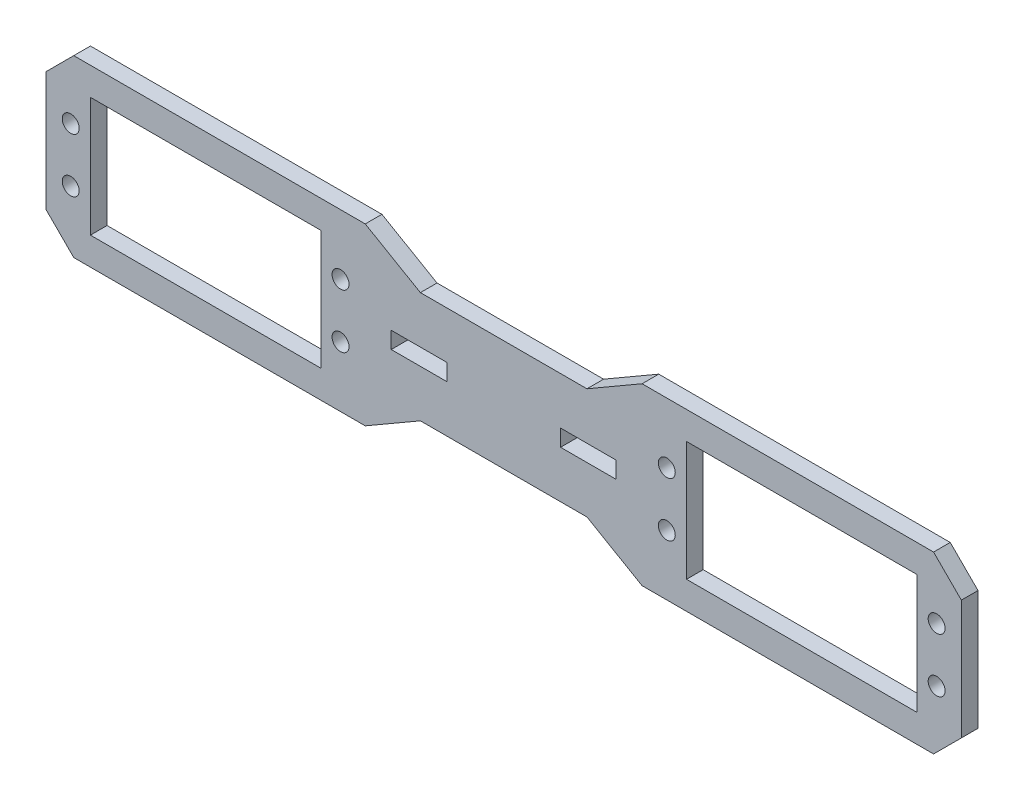
SolidWorks part; units mm, degrees
ref_plane "前视基准面" through (0, 0, 0) normal (0, 0, 1) x (1, 0, 0)
ref_plane "上视基准面" through (0, 0, 0) normal (0, 1, 0) x (1, 0, 0)
ref_plane "右视基准面" through (0, 0, 0) normal (1, 0, 0) x (0, 0, -1)
other "Configuration Table"
sketch "草图1" plane through (0, 0, 0) normal (0, 0, 1) x (1, 0, 0)
  line L0 (-68.821, 0) -> (77.2988, 0) construction
  line L1 (0, 51.7992) -> (0, -44.0645) construction
  line L2 (-77.2745, 15.6597) -> (-82.2745, 10.6597)
  line L3 (-77.2745, -15.8403) -> (-24.7745, -15.8403)
  line L4 (-82.2745, -10.8403) -> (-82.2745, 10.6597)
  line L5 (-77.2745, 15.6597) -> (-24.7745, 15.6597)
  line L6 (82.5855, -10.8403) -> (82.5855, 10.6597)
  line L7 (-32.7745, 10.6597) -> (-74.2745, 10.6597)
  line L8 (33.0855, -10.8403) -> (74.5855, -10.8403)
  line L9 (-82.2745, -10.8403) -> (-77.2745, -15.8403)
  line L10 (77.5855, -15.8403) -> (82.5855, -10.8403)
  line L11 (82.5855, 10.6597) -> (77.5855, 15.6597)
  line L12 (33.0855, -10.8403) -> (33.0855, 10.6597)
  line L13 (33.0855, 10.6597) -> (74.5855, 10.6597)
  line L14 (74.5855, -10.8403) -> (74.5855, 10.6597)
  line L15 (-74.2745, -10.8403) -> (-74.2745, 10.6597)
  line L16 (-32.7745, -10.8403) -> (-74.2745, -10.8403)
  line L17 (-32.7745, -10.8403) -> (-32.7745, 10.6597)
  line L18 (78.1355, -4.9653) -> (78.1355, 4.7847)
  line L19 (-24.7745, 15.6597) -> (-14.8445, 9.9097)
  line L20 (-14.8445, 9.9097) -> (15.1555, 9.9097)
  line L21 (15.1555, 9.9097) -> (25.0855, 15.6597)
  line L22 (15.1555, -10.0903) -> (25.0855, -15.8403)
  line L23 (-14.8445, -10.0903) -> (15.1555, -10.0903)
  line L24 (-24.7745, -15.8403) -> (-14.8445, -10.0903)
  line L25 (20.4036, 1.4097) -> (10.4036, 1.4097)
  line L26 (-20.0925, -1.5903) -> (-10.0925, -1.5903)
  line L27 (-20.0925, -1.5903) -> (-20.0925, 1.4097)
  line L28 (-20.0925, 1.4097) -> (-10.0925, 1.4097)
  line L29 (-10.0925, -1.5903) -> (-10.0925, 1.4097)
  line L30 (10.4036, -1.5903) -> (10.4036, 1.4097)
  line L31 (20.4036, -1.5903) -> (10.4036, -1.5903)
  line L32 (20.4036, -1.5903) -> (20.4036, 1.4097)
  line L33 (25.0855, 15.6597) -> (77.5855, 15.6597)
  line L34 (25.0855, -15.8403) -> (77.5855, -15.8403)
  circle A0 centre (78.1355, 4.7847) radius 1.525
  circle A1 centre (78.1355, -4.9653) radius 1.525
  circle A2 centre (-77.8245, -4.9653) radius 1.525
  circle A3 centre (-77.8245, 4.7847) radius 1.525
  circle A4 centre (29.5355, 4.7847) radius 1.525
  circle A5 centre (29.5355, -4.9653) radius 1.525
  circle A6 centre (-29.2245, -4.9653) radius 1.525
  circle A7 centre (-29.2245, 4.7847) radius 1.525
  point P6 (0.1555, -0.0903)
  point P37 (0.1555, -0.0903)
  dimension "D7" = 3.05
  dimension "D8" = 3.05
  dimension "D1" = 45
  dimension "D2" = 41.5
  dimension "D3" = 8
  dimension "D4" = 5
  dimension "D5" = 9.75
  dimension "D6" = 4.45
  dimension "D9" = 9.75
  dimension "D10" = 48.6
  dimension "D11" = 164.86
  dimension "D12" = 31.5
  dimension "D13" = 5.75
  dimension "D14" = 57.5
  dimension "D15" = 30
  dimension "D16" = 21.5
  dimension "D17" = 3
  dimension "D18" = 10
  dimension "D19" = 20.496
extrude "凸台-拉伸3" add sketch "草图1" along normal blind 3
